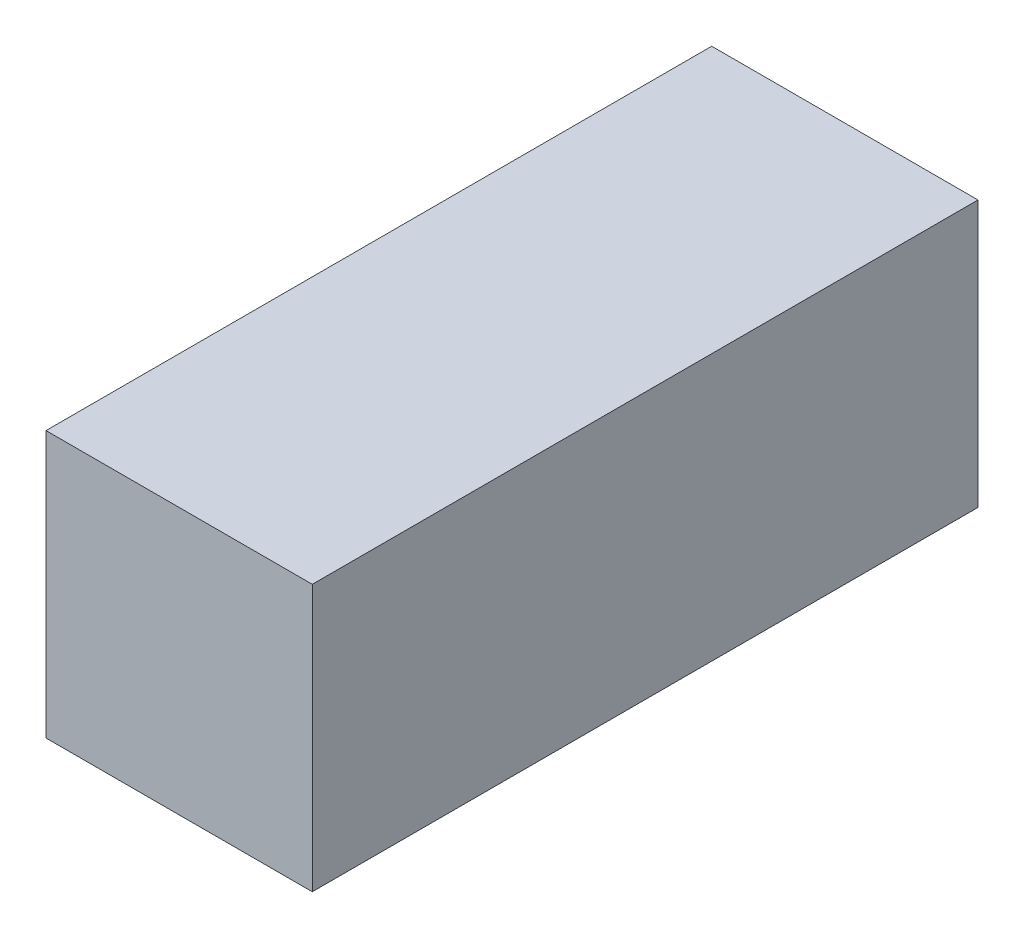
SolidWorks part; units mm, degrees
material "普通碳钢"
ref_plane "Front Plane" through (0, 0, 0) normal (0, 0, 1) x (1, 0, 0)
ref_plane "Top Plane" through (0, 0, 0) normal (0, 1, 0) x (1, 0, 0)
ref_plane "Right Plane" through (0, 0, 0) normal (1, 0, 0) x (0, 0, -1)
sketch "Sketch1" plane through (0, 0, 0) normal (0, 0, 1) x (1, 0, 0)
  line L1 (-40, 40) -> (40, 40)
  line L2 (-40, 40) -> (-40, -40)
  line L3 (-40, -40) -> (40, -40)
  line L4 (40, 40) -> (40, -40)
  point P0 (0, 0)
  dimension "D1" = 80
  dimension "D2" = 80
extrude "Boss-Extrude1" add sketch "Sketch1" along normal mid plane 200
